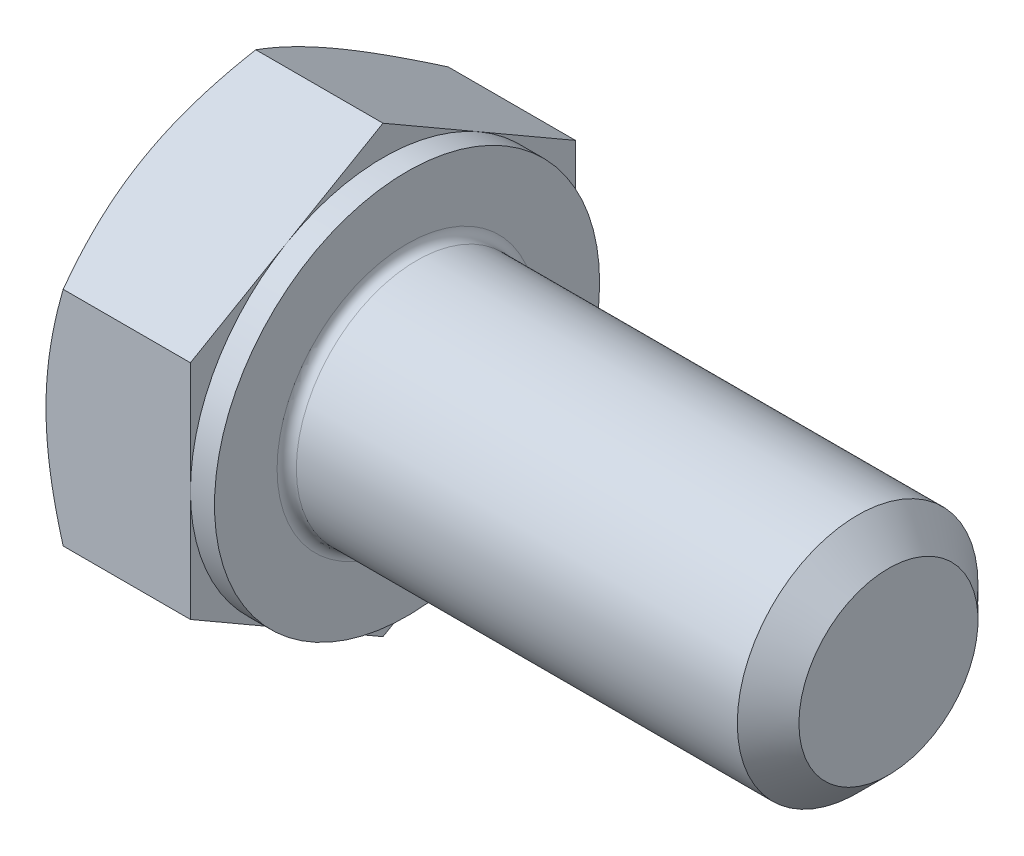
from build123d import *

# Parameters (mm, degrees)
BASE_EXTRUDE_DEPTH = 3.5
SKETCH4_W          = 0.5
SKETCH4_H          = 10.618802154
CHAMFER_2_SIZE     = 0.64
FILLET_2_R         = 0.2


with BuildPart() as part:
    # Sketch1 → Base-Extrude (new body)
    with BuildSketch(Plane(origin=(0, 0, 0), x_dir=(0, 0, -1), z_dir=(1, 0, 0))):
        Polygon((4, 2.309401077), (4, -2.309401077), (0, -4.618802154), (-4, -2.309401077), (-4, 2.309401077), (0, 4.618802154), align=None)
    extrude(amount=BASE_EXTRUDE_DEPTH)

    # Sketch2 → Boss-Revolve1 (revolve)
    with BuildSketch(Plane.XY, mode=Mode.PRIVATE) as boss_revolve1_sk:
        Polygon((0, 0), (13.5, 0), (13.5, 1.8072), (13.5, 2.5), (0, 2.5), align=None)
    revolve(boss_revolve1_sk.sketch.rotate(Axis((0, 0, 0), (1, 0, 0)), 90), axis=Axis((0, 0, 0), (1, 0, 0)))

    # Sketch3 → Cut-Revolve1 (revolve, cut)
    with BuildSketch(Plane.XY):
        Polygon((0, 4), (3.244016936, 9.618802154), (3.244016936, 14.618802154), (-10, 14.618802154), (-10, 4), align=None)
    revolve(axis=Axis((0, 0, 0), (1, 0, 0)), mode=Mode.SUBTRACT)

    # Sketch5 → Cut-Revolve2 (revolve, cut)
    with BuildSketch(Plane.XY):
        Polygon((3.5, 4), (0.255983064, 9.618802154), (0.255983064, 14.618802154), (10.255983064, 14.618802154), (10.255983064, 4), align=None)
    revolve(axis=Axis((0, 0, 0), (1, 0, 0)), mode=Mode.SUBTRACT)

    # Sketch4 → Cut-Revolve3 (revolve, cut)
    with BuildSketch(Plane.XY, mode=Mode.PRIVATE) as cut_revolve3_sk:
        with Locations((3.25, 9.309401077)):
            Rectangle(SKETCH4_W, SKETCH4_H)
    revolve(cut_revolve3_sk.sketch.rotate(Axis((0, 0, 0), (1, 0, 0)), 270), axis=Axis((0, 0, 0), (1, 0, 0)), mode=Mode.SUBTRACT)

    # Chamfer 2
    chamfer_2_edges = [part.edges().sort_by_distance(p)[0] for p in [
        (13.5, 0, -2.5),
    ]]
    chamfer(chamfer_2_edges, length=CHAMFER_2_SIZE)

    # Fillet 2
    fillet_2_edges = [part.edges().sort_by_distance(p)[0] for p in [
        (3.5, 0, -2.5),
    ]]
    fillet(fillet_2_edges, radius=FILLET_2_R)


solid = part.part
